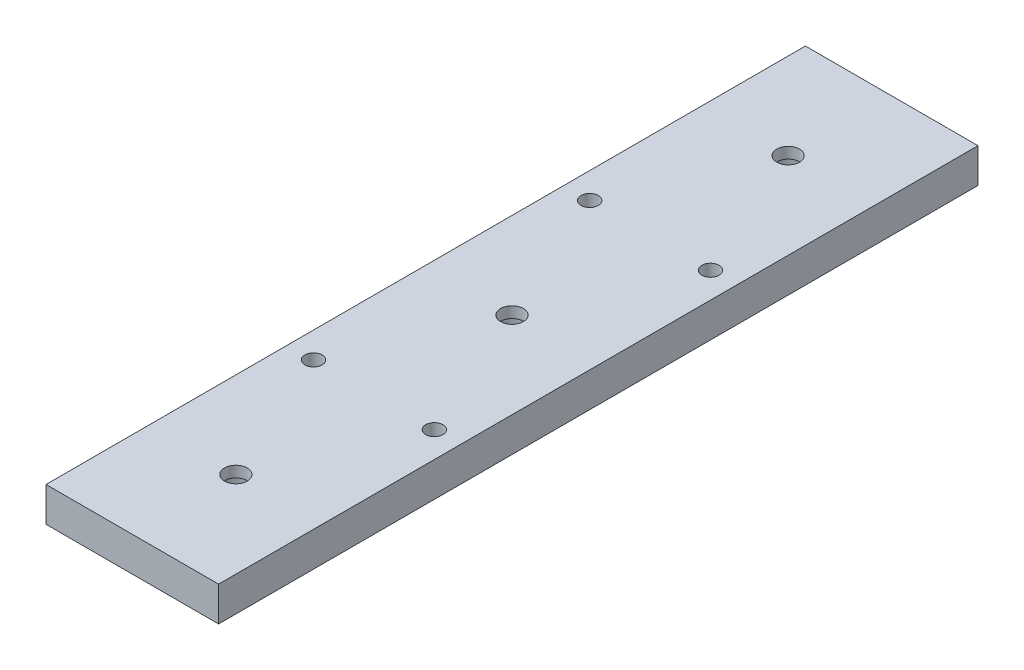
from build123d import *

# Parameters (mm, degrees)
SKETCH1_W                                         = 50
SKETCH1_H                                         = 220
BOSS_EXTRUDE1_DEPTH                               = 10
HOLE_SIZE_BY_SOCKET_HEAD_CAP_SCREW_TY_D           = 6.6
HOLE_SIZE_BY_SOCKET_HEAD_CAP_SCREW_TY_CBORE_D     = 11
HOLE_SIZE_BY_SOCKET_HEAD_CAP_SCREW_TY_CBORE_DEPTH = 6.8
M6_TAPPED_HOLE1_D                                 = 5
M6_TAPPED_HOLE1_DEPTH                             = 15
M6_TAPPED_HOLE1_TIP                               = 1.502151548


with BuildPart() as part:
    # Sketch1 → Boss-Extrude1 (new body)
    with BuildSketch(Plane(origin=(0, 0, 0), x_dir=(1, 0, 0), z_dir=(0, 1, 0))):
        Rectangle(SKETCH1_W, SKETCH1_H)
    extrude(amount=BOSS_EXTRUDE1_DEPTH)

    # Hole Size (% by) Socket Head Cap Screw Type1 (through all)
    with Locations(Plane(origin=(0, 0, 0), x_dir=(-1, 0, 0), z_dir=(0, -1, 0))):
        with Locations((0, -80), (0, 80), (0, 0)):
            CounterBoreHole(HOLE_SIZE_BY_SOCKET_HEAD_CAP_SCREW_TY_D / 2, HOLE_SIZE_BY_SOCKET_HEAD_CAP_SCREW_TY_CBORE_D / 2, HOLE_SIZE_BY_SOCKET_HEAD_CAP_SCREW_TY_CBORE_DEPTH)

    # M6 Tapped Hole1
    with Locations(Plane(origin=(0, 10, 0), x_dir=(1, 0, 0), z_dir=(0, 1, 0))):
        with Locations((-17.5, 40), (-17.5, -40), (17.5, 40), (17.5, -40)):
            Hole(M6_TAPPED_HOLE1_D / 2, depth=M6_TAPPED_HOLE1_DEPTH)
            with Locations((0, 0, -(M6_TAPPED_HOLE1_DEPTH + M6_TAPPED_HOLE1_TIP / 2))):  # 118° drill point
                Cone(0, M6_TAPPED_HOLE1_D / 2, M6_TAPPED_HOLE1_TIP, mode=Mode.SUBTRACT)


solid = part.part
